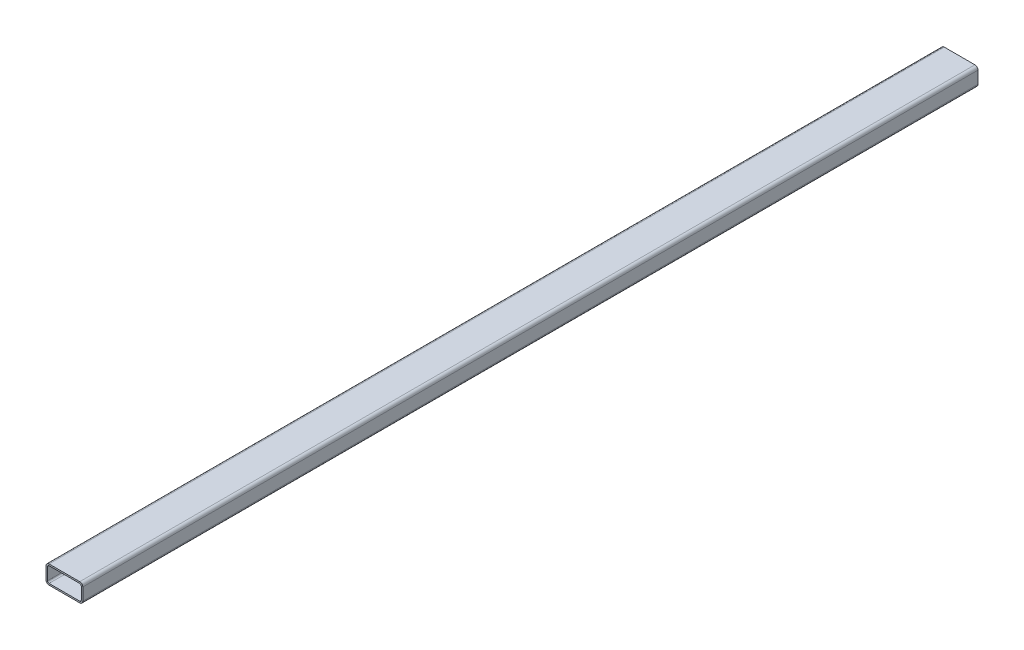
from build123d import *

# Parameters (mm, degrees)
BOSS_EXTRUDE1_DEPTH = 2920


with BuildPart() as part:
    # Sketch1 → Boss-Extrude1 (new body)
    with BuildSketch(Plane.XY):
        with BuildLine():
            Line((10, 0), (110, 0))
            ThreePointArc((110, 0), (117.071067812, 2.928932188), (120, 10))
            Line((120, 10), (120, 50))
            ThreePointArc((120, 50), (117.071067812, 57.071067812), (110, 60))
            Line((110, 60), (10, 60))
            ThreePointArc((10, 60), (2.928932188, 57.071067812), (0, 50))
            Line((0, 50), (0, 10))
            ThreePointArc((0, 10), (2.928932188, 2.928932188), (10, 0))
        make_face()
        with BuildLine():
            Line((10, 55), (110, 55))
            ThreePointArc((110, 55), (113.535533906, 53.535533906), (115, 50))
            Line((115, 50), (115, 10))
            ThreePointArc((115, 10), (113.535533906, 6.464466094), (110, 5))
            Line((110, 5), (10, 5))
            ThreePointArc((10, 5), (6.464466094, 6.464466094), (5, 10))
            Line((5, 10), (5, 50))
            ThreePointArc((5, 50), (6.464466094, 53.535533906), (10, 55))
        make_face(mode=Mode.SUBTRACT)
    extrude(amount=BOSS_EXTRUDE1_DEPTH)


solid = part.part
